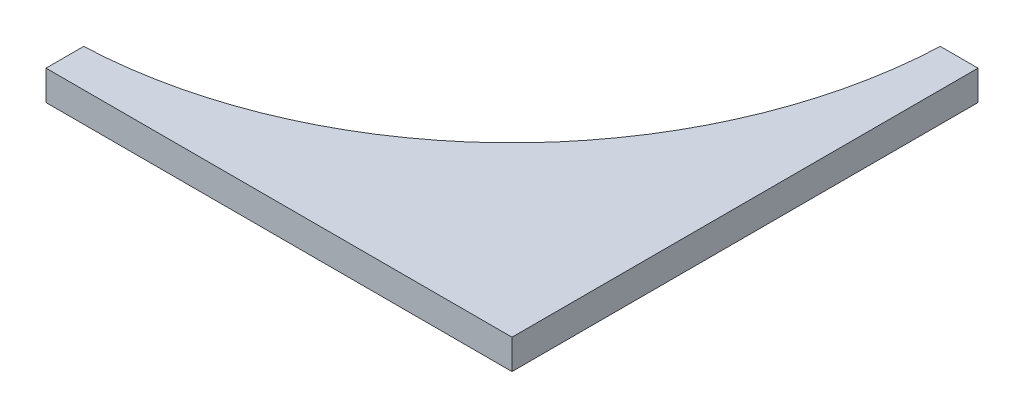
from build123d import *

# Parameters (mm, degrees)
EXTRUDE_1_DEPTH = 8


with BuildPart() as part:
    # 草图1 → 凸台-拉伸1 (new body)
    with BuildSketch(Plane(origin=(0, 0, 0), x_dir=(1, 0, 0), z_dir=(0, 1, 0))):
        with BuildLine():
            Line((-125, 0), (0, 0))
            Line((0, 0), (0, 125))
            Line((0, 125), (-10.104211917, 125))
            ThreePointArc((-10.104211917, 125), (-45.147186258, 45.147186258), (-125, 10.104211917))
            Line((-125, 10.104211917), (-125, 0))
        make_face()
    extrude(amount=EXTRUDE_1_DEPTH)


solid = part.part
